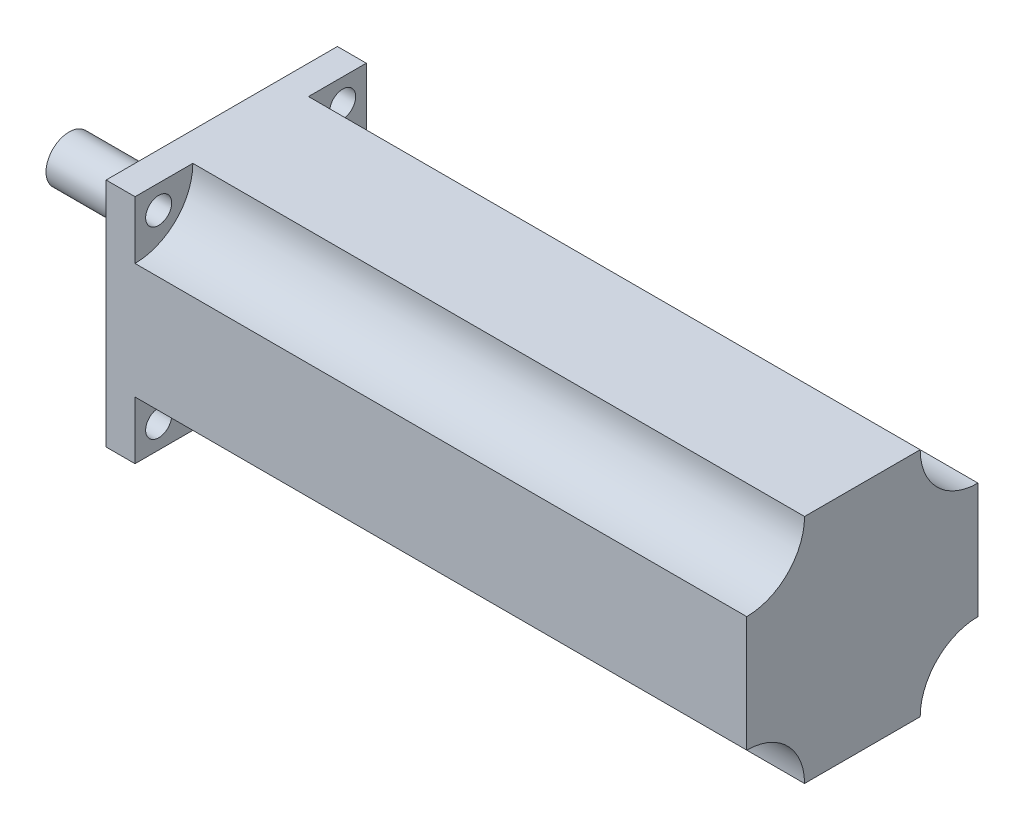
SolidWorks part; units mm, degrees
material "6061"
ref_plane "Front Plane" through (0, 0, 0) normal (0, 0, 1) x (1, 0, 0)
ref_plane "Top Plane" through (0, 0, 0) normal (0, 1, 0) x (1, 0, 0)
ref_plane "Right Plane" through (0, 0, 0) normal (1, 0, 0) x (0, 0, -1)
sketch "Sketch1" plane through (0, 0, 0) normal (0, 0, 1) x (1, 0, 0)
  line L1 (-55.4, 20) -> (55.4, 20)
  line L2 (-55.4, 20) -> (-55.4, -20)
  line L3 (-55.4, -20) -> (55.4, -20)
  line L4 (55.4, 20) -> (55.4, -20)
  line L5 (-55.4, 20) -> (55.4, -20) construction
  line L6 (-55.4, -20) -> (55.4, 20) construction
  point P0 (0, 0)
  dimension "D1" = 40
  dimension "D2" = 110.8
extrude "Boss-Extrude1" add sketch "Sketch1" along normal blind 40
sketch "Sketch2" plane through (-55.4, 0, 0) normal (-1, 0, 0) x (0, 0, 1)
  line L0 (20, 20) -> (20, -20) construction
  line L1 (40, 20) -> (0, 20) construction
  line L2 (40, -20) -> (0, -20) construction
  circle A0 centre (20, 0) radius 15
  dimension "D1" = 30
extrude "Boss-Extrude2" add sketch "Sketch2" along normal blind 2.6
sketch "Sketch3" plane through (-58, 0, 0) normal (-1, 0, 0) x (0, 0, 1)
  circle A0 centre (20, 0) radius 4
  dimension "D1" = 8
extrude "Boss-Extrude3" add sketch "Sketch3" along normal blind 23.8
sketch "Sketch4" plane through (55.4, 0, 0) normal (1, 0, 0) x (0, 0, -1)
  circle A0 centre (-40, 20) radius 10
  circle A1 centre (0, 20) radius 10
  circle A2 centre (-40, -20) radius 10
  circle A3 centre (0, -20) radius 10
  dimension "D1" = 20
extrude "Cut-Extrude1" cut sketch "Sketch4" against normal blind 105.8
hole_wizard "M4 Clearance Hole1" positions "Sketch6" profile "Sketch5" hole size "M4" standard "Iso"
sketch "Sketch6" plane through (-55.4, 0, 0) normal (-1, 0, 0) x (0, 0, 1)
  line L0 (20, 0) -> (4.0901, 15.9099) construction
  line L3 (20, 0) -> (20, 20) construction
  line L4 (40, 20) -> (0, 20) construction
  point P0 (4.0901, 15.9099)
  dimension "D1" = 45
  dimension "D2" = 22.5
sketch "Sketch5" plane through (-55.4, 15.9099, 4.0901) normal (0, 1, 0) x (0, 0, 1)
  line L0 (0, 0) -> (0, 258.8519)
  line L1 (0, 258.8519) -> (2.25, 257.5)
  line L2 (2.25, 257.5) -> (2.25, 0)
  line L5 (2.25, 0) -> (0, 0)
  line L10 (0, 258.8519) -> (-2.25, 257.5) construction
  line L11 (0, -6.35) -> (0, 107.95) construction
  dimension "孔直径" = 4.5
  dimension "孔深度" = 257.5
  dimension "导头角度" = 118
pattern_circular "CirPattern1" count 4 over 360 about axis through (0, 0, 20) along (1, 0, 0) of "M4 Clearance Hole1"
